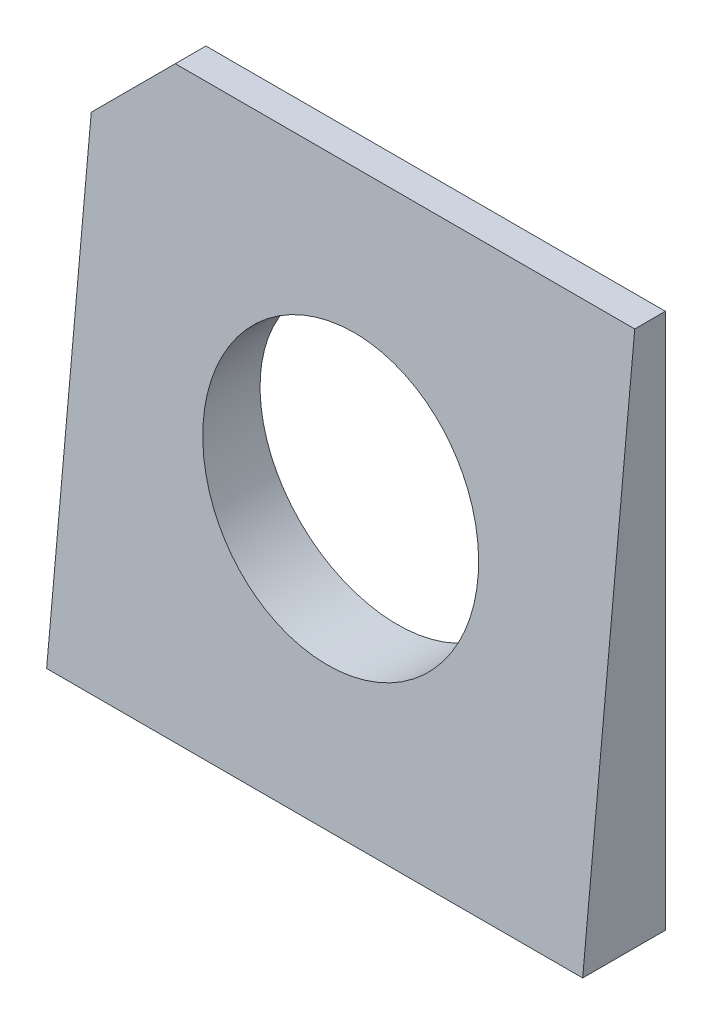
SolidWorks part; units mm, degrees
ref_plane "Front" through (0, 0, 0) normal (0, 0, 1) x (1, 0, 0)
ref_plane "Top" through (0, 0, 0) normal (0, 1, 0) x (1, 0, 0)
ref_plane "Right" through (0, 0, 0) normal (1, 0, 0) x (0, 0, -1)
sketch "Dimension Sketch" plane through (0, 0, 0) normal (0, 0, 1) x (1, 0, 0)
  line L0 (0, 0) -> (35, 0) construction
  point P2 (17.93, 0)
  point P3 (35, 0)
  point P4 (2, 0)
  point P5 (5.4, 0)
  dimension "d" = 17.93
  dimension "B" = 35
  dimension "H" = 2
  dimension "H1" = 5.4
sketch "Sketch1" plane through (0, 0, 0) normal (0, 0, 1) x (1, 0, 0)
  line L0 (0, 0) -> (0, -17.5) construction
  line L1 (-17.5, 17.5) -> (17.5, 17.5)
  line L2 (-17.5, 17.5) -> (-17.5, -17.5)
  line L3 (-17.5, -17.5) -> (17.5, -17.5)
  line L4 (17.5, 17.5) -> (17.5, -17.5)
  line L5 (17.5, 0) -> (-17.5, 0) construction
  circle A0 centre (0, 0) radius 8.965
  dimension "d" = 17.93
  dimension "B" = 35
  dimension "B." = 35
extrude "Boss-Extrude" add sketch "Sketch1" along normal blind 5.4
sketch "Sketch2" plane through (17.5, 0, 0) normal (1, 0, 0) x (0, 0, -1)
  line L0 (-5.4, -17.5) -> (-2, 17.5)
  line L4 (0, -17.5) -> (0, 17.5)
  line L5 (0, 17.5) -> (-5.4, 17.5)
  line L6 (-5.4, 17.5) -> (-5.4, -17.5)
  line L7 (-5.4, -17.5) -> (0, -17.5)
  line L8 (0, -17.5) -> (0, 17.5)
  line L9 (0, 17.5) -> (-2, 17.5)
  line L11 (-5.4, -17.5) -> (0, -17.5)
  dimension "H" = 2
  dimension "D1" = 0
extrude "Cut-Extrude1" cut sketch "Sketch2" against normal up to surface (35 mm away) flip side to cut up to face at (-17.5, 0, 2.7)
sketch "Sketch3" plane through (0, 0, 0) normal (0, 0, -1) x (-1, 0, 0)
  line L0 (12.5, 17.5) -> (17.5, 12.5)
  line L4 (17.5, -17.5) -> (17.5, 17.5)
  line L5 (17.5, 17.5) -> (-17.5, 17.5)
  line L6 (-17.5, 17.5) -> (-17.5, -17.5)
  line L7 (-17.5, -17.5) -> (17.5, -17.5)
  line L8 (17.5, 12.5) -> (17.5, 17.5)
  line L9 (17.5, 17.5) -> (12.5, 17.5)
  dimension "D2" = 5
  dimension "D3" = 5
  dimension "D1" = 0
extrude "Cut-Extrude2" cut sketch "Sketch3" against normal through all
